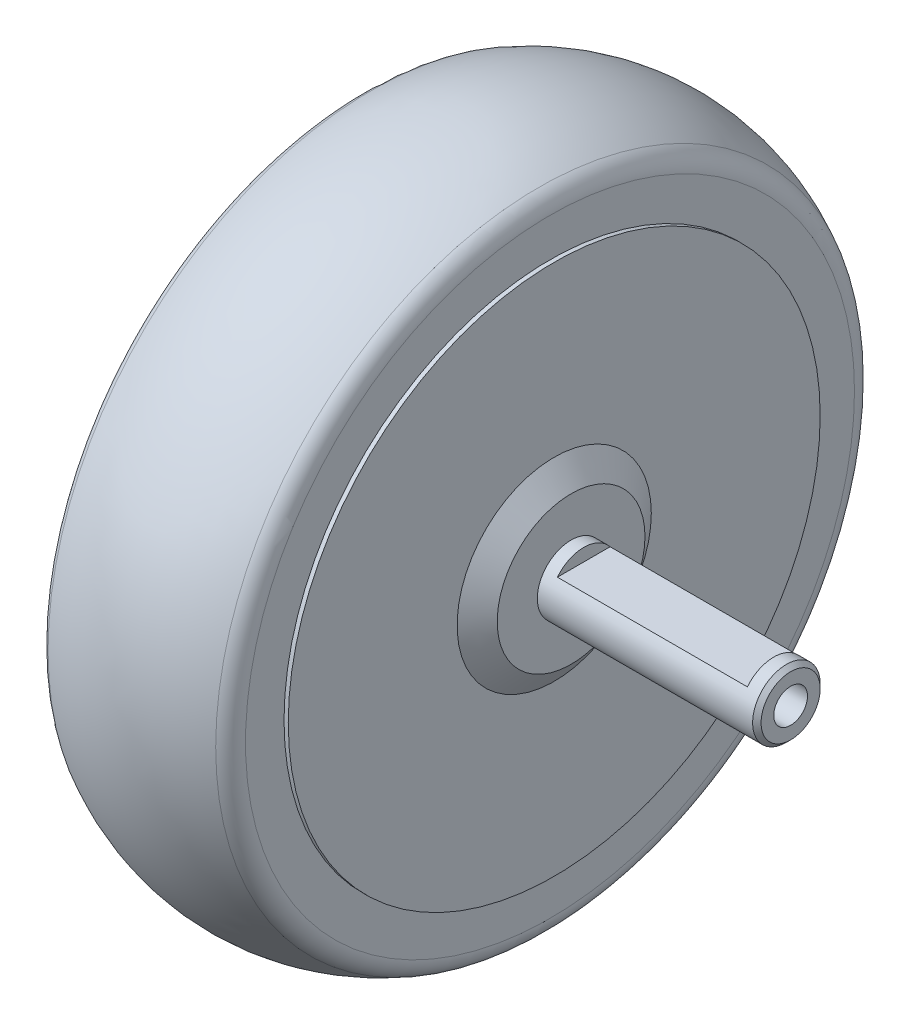
from build123d import *

# Parameters (mm, degrees)
FILLET1_R          = 5
CUT_EXTRUDE2_START = -4
CUT_EXTRUDE2_DEPTH = 45
CHAMFER1_SIZE      = 1
SKETCH4_R          = 4
CUT_EXTRUDE3_DEPTH = 50


with BuildPart() as part:
    # Sketch1 → Revolve1 (revolve)
    with BuildSketch(Plane.XY, mode=Mode.PRIVATE) as revolve1_sk:
        with BuildLine():
            Line((19.577327609, 0), (19.577327609, 50))
            Line((19.577327609, 50), (29.577327609, 57))
            Line((29.577327609, 57), (29.577327609, 75))
            ThreePointArc((29.577327609, 75), (52.077327609, 81.5), (74.577327609, 75))
            Line((74.577327609, 75), (74.577327609, 63))
            Line((74.577327609, 63), (75.577327609, 63))
            Line((75.577327609, 63), (75.577327609, 23))
            Line((75.577327609, 23), (79.577327609, 17.5))
            Line((79.577327609, 17.5), (79.577327609, 8))
            Line((79.577327609, 8), (131.577327609, 8))
            Line((131.577327609, 8), (131.577327609, 0))
            Line((131.577327609, 0), (19.577327609, 0))
        make_face()
    revolve(revolve1_sk.sketch.rotate(Axis((0, 0, 0), (-1, 0, 0)), 90), axis=Axis((0, 0, 0), (-1, 0, 0)))

    # Fillet1
    fillet1_edges = [part.edges().sort_by_distance(p)[0] for p in [
        (74.577327609, 0, 75),
        (29.577327609, 0, 75),
    ]]
    fillet(fillet1_edges, radius=FILLET1_R)

    # Sketch3 → Cut-Extrude2 (cut)
    with BuildSketch(Plane(origin=(131.577327609, 0, 0), x_dir=(0, 0, -1), z_dir=(1, 0, 0)).offset(CUT_EXTRUDE2_START)):
        with BuildLine():
            Line((-6.244997998, 5), (6.244997998, 5))
            ThreePointArc((6.244997998, 5), (0, 8), (-6.244997998, 5))
        make_face()
    extrude(amount=-CUT_EXTRUDE2_DEPTH, mode=Mode.SUBTRACT)

    # Chamfer1
    chamfer1_edges = [part.edges().sort_by_distance(p)[0] for p in [
        (131.577327609, 0, 8),
    ]]
    chamfer(chamfer1_edges, length=CHAMFER1_SIZE)

    # Sketch4 → Cut-Extrude3 (cut)
    with BuildSketch(Plane(origin=(131.577327609, 0, 0), x_dir=(0, 0, -1), z_dir=(1, 0, 0))):
        Circle(SKETCH4_R)
    extrude(amount=-CUT_EXTRUDE3_DEPTH, mode=Mode.SUBTRACT)


solid = part.part
